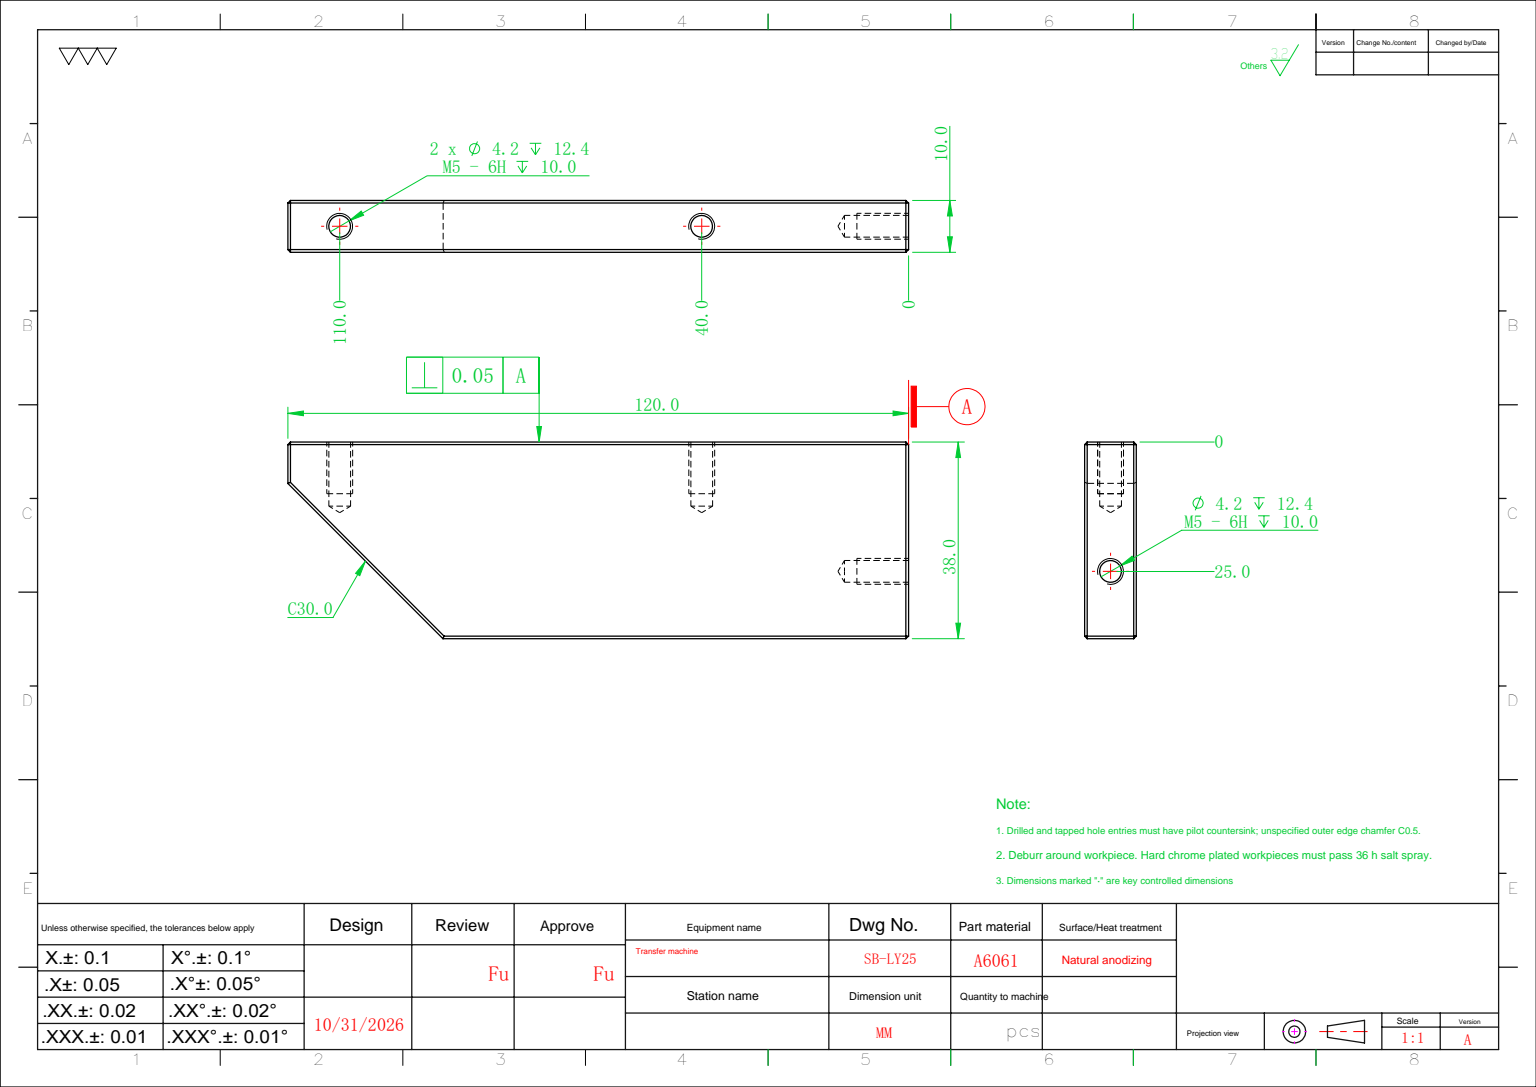
SolidWorks part; units mm, degrees
ref_plane "前视基准面" through (0, 0, 0) normal (0, 0, 1) x (1, 0, 0)
ref_plane "上视基准面" through (0, 0, 0) normal (0, 1, 0) x (1, 0, 0)
ref_plane "右视基准面" through (0, 0, 0) normal (1, 0, 0) x (0, 0, -1)
sketch "草图1" plane through (0, 0, 0) normal (0, 0, 1) x (1, 0, 0)
  line L1 (-60, -19) -> (60, -19)
  line L2 (-60, -19) -> (-60, 19)
  line L3 (-60, 19) -> (60, 19)
  line L4 (60, -19) -> (60, 19)
  line L5 (-60, -19) -> (60, 19) construction
  line L6 (-60, 19) -> (60, -19) construction
  point P0 (0, 0)
  dimension "D1" = 120
  dimension "D2" = 38
extrude "凸台-拉伸1" add sketch "草图1" along normal blind 10
chamfer "倒角1" distance 30 angle 45 1 edges at (60, 19, 5)
hole_wizard "M5 螺纹孔1" positions "草图2" profile "草图3" tap size "M5" standard "ISO"
sketch "草图2" plane through (-60, 0, 0) normal (-1, 0, 0) x (0, 0, 1)
  line L0 (5, -19) -> (5, 19) construction
  line L1 (10, -19) -> (0, -19) construction
  line L2 (10, 19) -> (0, 19) construction
  point P0 (5, 6)
  dimension "D1" = 25
sketch "草图3" plane through (-60, 6, 5) normal (0, 1, 0) x (0, 0, 1)
  line L0 (0, 0) -> (0, 13.6618)
  line L1 (0, 13.6618) -> (2.1, 12.4)
  line L2 (2.1, 12.4) -> (2.1, 0)
  line L5 (2.1, 0) -> (0, 0)
  line L10 (0, 13.6618) -> (-2.1, 12.4) construction
  line L11 (0, -6.35) -> (0, 107.95) construction
  dimension "螺纹孔钻头直径" = 4.2
  dimension "螺纹孔钻头深度" = 12.4
  dimension "导头角度" = 118
cosmetic thread "孔螺蚊线1" parameters "D1"=10, "D2"=5
hole_wizard "M5 螺纹孔2" positions "草图4" profile "草图5" tap size "M5" standard "ISO"
sketch "草图4" plane through (0, -19, 0) normal (0, -1, 0) x (-1, 0, 0)
  line L0 (60, -5) -> (-66.4875, -5) construction
  line L1 (60, -10) -> (60, 0) construction
  point P0 (-50, -5)
  point P3 (20, -5)
  dimension "D1" = 40
  dimension "D2" = 70
sketch "草图5" plane through (50, -19, 5) normal (1, 0, 0) x (0, 0, -1)
  line L0 (0, 0) -> (0, 13.6618)
  line L1 (0, 13.6618) -> (2.1, 12.4)
  line L2 (2.1, 12.4) -> (2.1, 0)
  line L5 (2.1, 0) -> (0, 0)
  line L10 (0, 13.6618) -> (-2.1, 12.4) construction
  line L11 (0, -6.35) -> (0, 107.95) construction
  dimension "螺纹孔钻头直径" = 4.2
  dimension "螺纹孔钻头深度" = 12.4
  dimension "导头角度" = 118
cosmetic thread "孔螺蚊线2" parameters "D1"=10, "D2"=5
cosmetic thread "孔螺蚊线3" parameters "D1"=10, "D2"=5
chamfer "倒角2" distance 0.5 angle 45 13 edges at (-60, -19, 5) (60, -19, 5) (0, -19, 10) (-60, 0, 10) (60, -15, 10) (45, 4, 10) (-15, 19, 10) (-60, 0, 0) (0, -19, 0) (60, -15, 0) (45, 4, 0) (-15, 19, 0) (-60, 19, 5)
